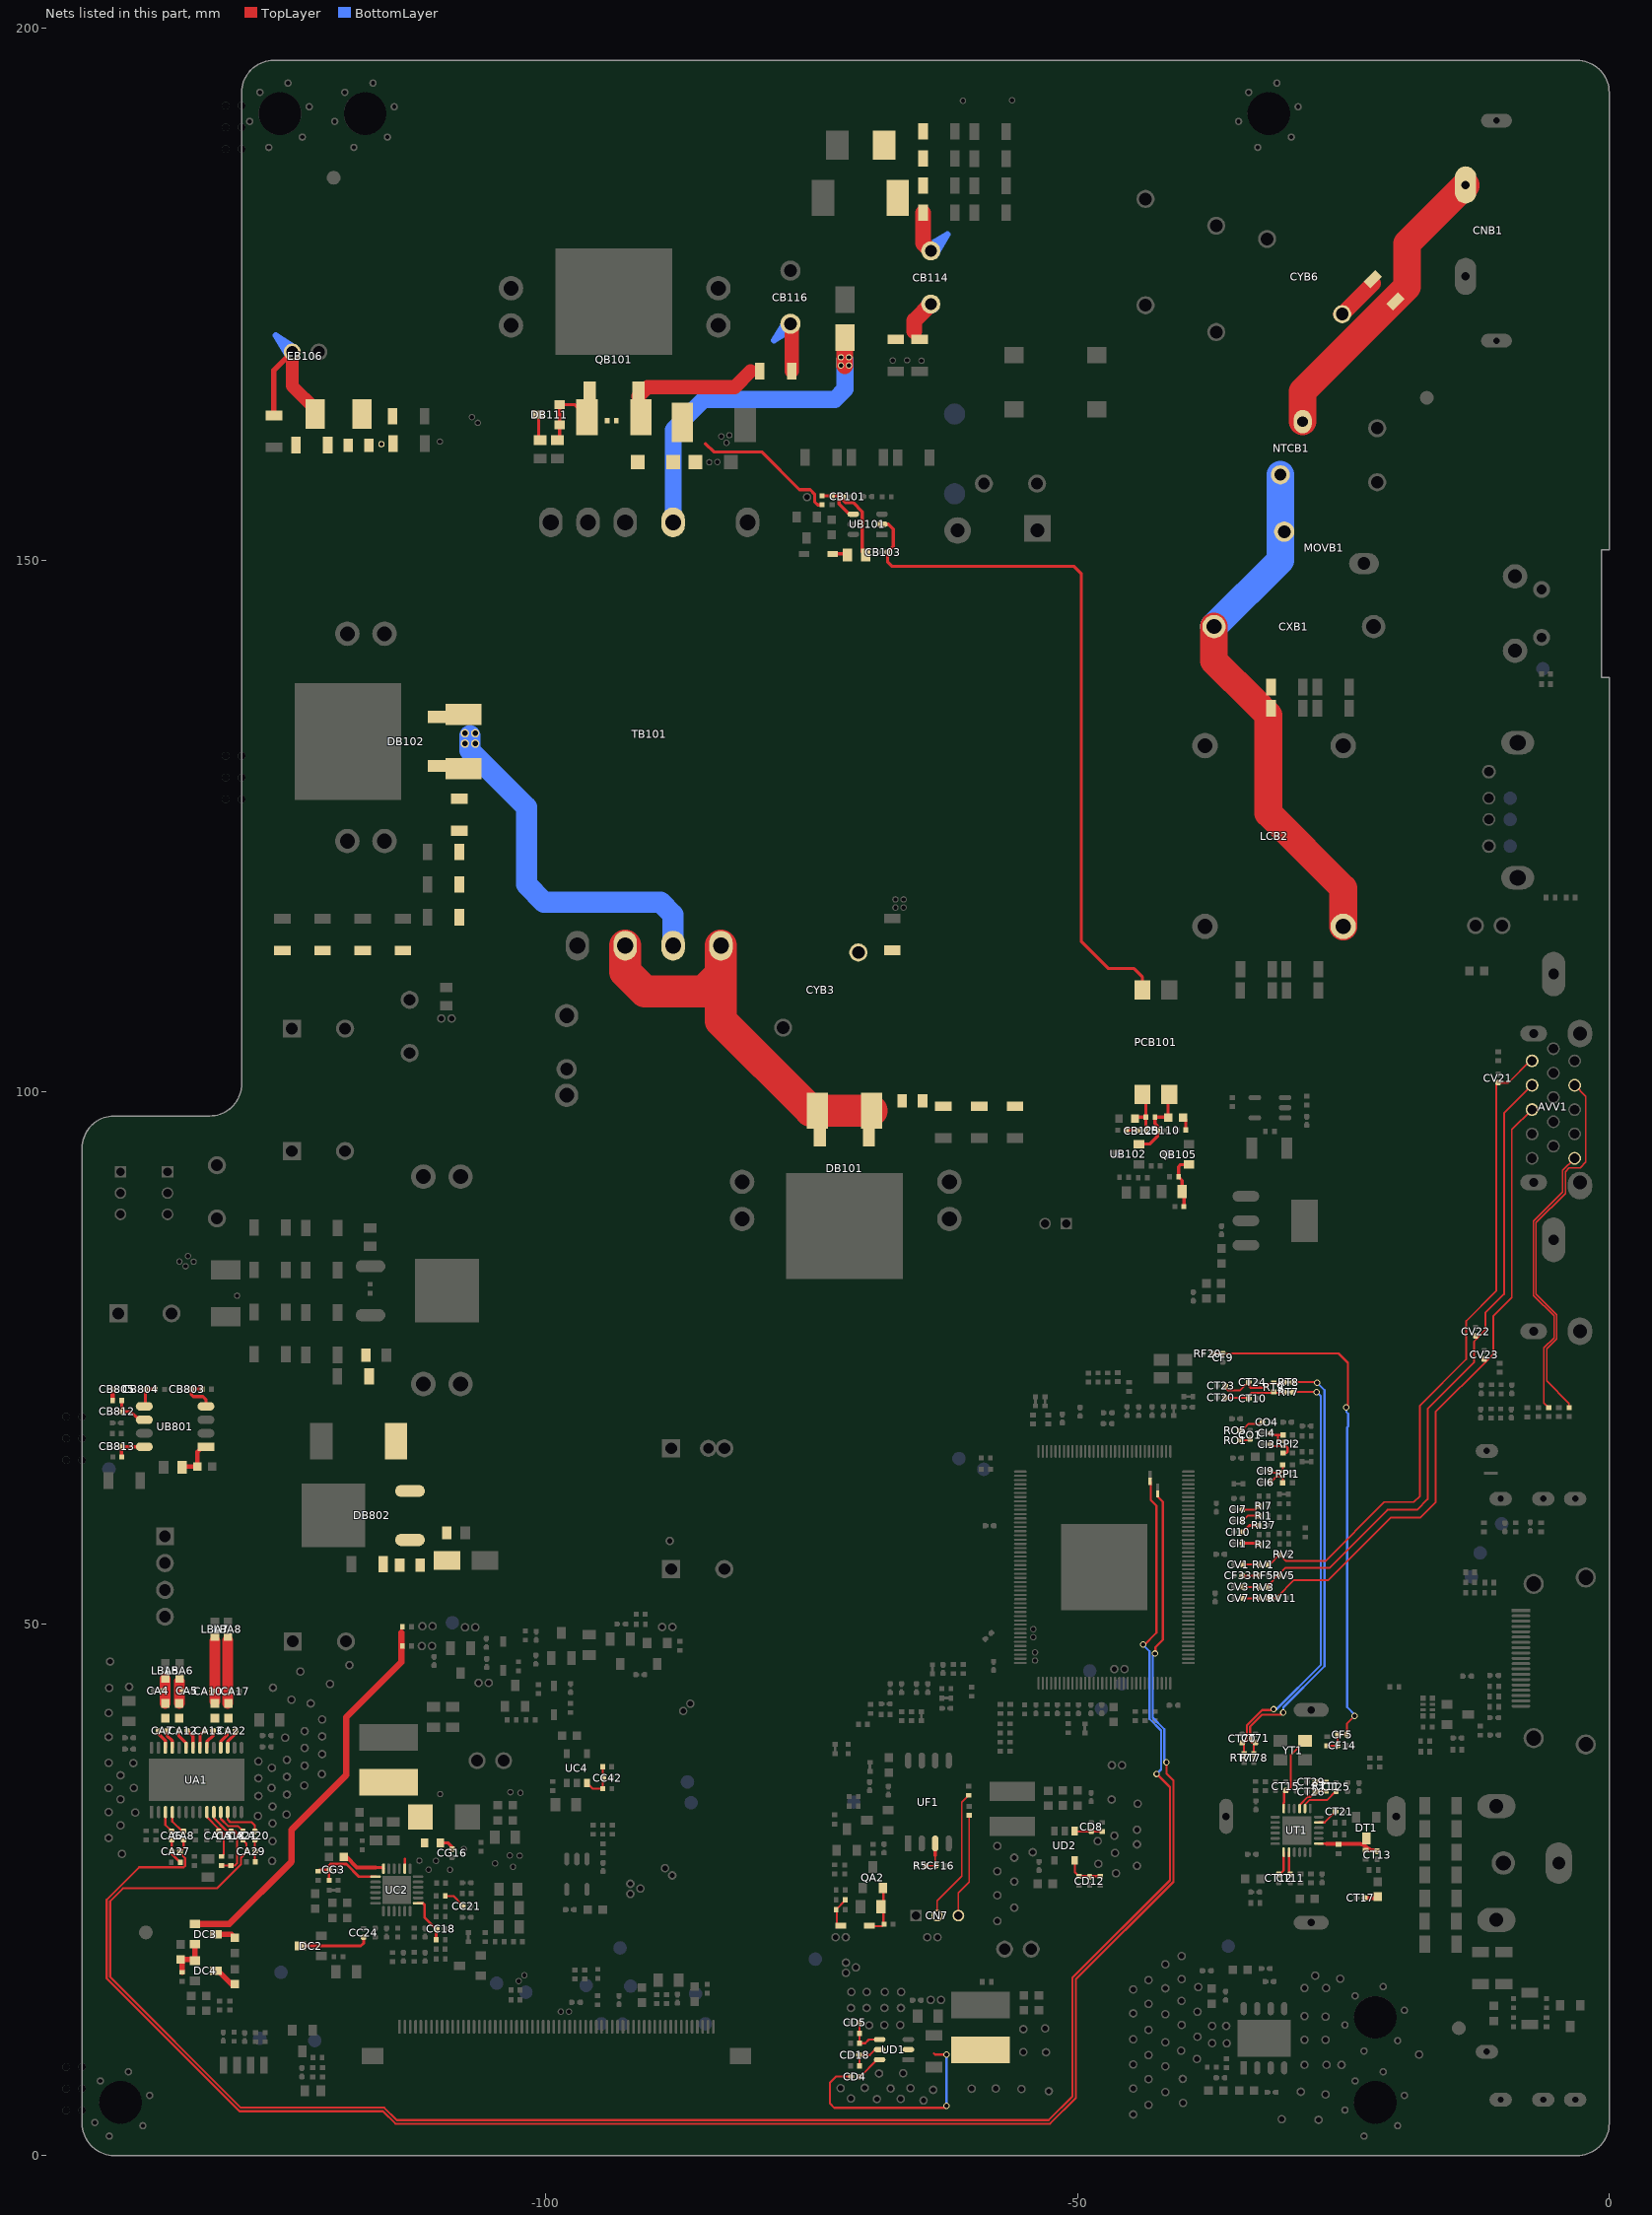
[diagram p0: the nets of this part, all layers, seen from the top]
# Altium PCB MISC86383-9.PcbDoc (part 13 of 18)
Units mm, origin at the board's own origin, x right, y up, seen from the top; angles counter-clockwise.
Board outline 143.6 x 197 mm, 2 copper layers (TopLayer, BottomLayer), stack 1.571 mm thick; 743 components, 401 nets, 2996 pads, 1077 vias.
Unrouted connection lines stored in the file: 4.

## Via types
v1: diameter 0.6, hole 0.4, TopLayer to BottomLayer, tented both sides, 993 vias
v2: diameter 0.6, hole 0.4, TopLayer to BottomLayer, 65 vias
v3: diameter 0.7, hole 0.5, TopLayer to BottomLayer, tented both sides, 15 vias
v4: diameter 0.8, hole 0.5, TopLayer to BottomLayer, tented both sides, 4 vias

## Nets (pads, with @x,y where several pads share a name; then routed paths per layer and width w, separated by ;. In a path a pad name is that pad's centre, name@x,y a point inside that pad or via, vN(x,y) a via of type N, cw(c..) or ccw(c..) an arc to the next point about the centre after c; other vN are vias at no path point) (continued)
N-1: CNB1.2 NTCB1.2@-28.82,163.041 RB160.1 | length 28.7
  TopLayer w2.6: NTCB1.2@-28.82,163.041 -28.82,165.883 -20.237,174.466 -19,175.704 -19,179.8 CNB1.2@-13.572,185.228 ; CNB1.2@-13.572,185.228 CNB1.2@-13.5,185.3 -13.5,185.228 CNB1.2@-13.572,185.228
N-2: CXB1.2 LCB2.1 MOVB1.2@-30.56,152.694 NTCB1.1 RB3.2 RB4.2 | length 50.1
  TopLayer w2.6: CXB1.2@-37.155,143.764 -37.155,140.558 -33.243,136.646 -32.24,135.643 -32.052,135.456 -32.052,126.21 -25.009,119.167 LCB2.1@-25.009,115.579
  BottomLayer w2.6: CXB1.2@-37.155,143.764 -30.92,149.998 -30.92,152.694 NTCB1.1@-30.92,158.041
N-3: CYB6.1 RB160.2 | length 4.2
  TopLayer w1.5: CYB6.1@-25.19,173.147 CYB6.1@-25.103,173.147 RB160.2@-22.219,176.031
NetAVV1_1: AVV1.1 CV21.2@-10.44,100.864 CV21.2@-10.44,101.039 RV1.2 RV2.2 | length 63.4
  TopLayer w0.175: RV1.2@-32.069,55.578 -31.92,55.578 RV2.2@-30.986,56.512 -30.379,55.905 -26.691,55.905 -21.153,61.444 -18.365,61.444 -17.799,62.01 -17.799,70.514 -13.446,74.867 -13.446,78.468 -10.624,81.29 -10.624,100.68 CV21.2@-10.44,100.864 -9.487,100.864 -7.351,103 AVV1.1@-7.351,103.03
  TopLayer w0.18: AVV1.1@-7.351,103.03 AVV1.1@-7.247,103.03
NetAVV1_2: AVV1.2 CV22.2@-12.56,77.22 CV22.2@-12.56,77.045 RV3.2 RV5.2 | length 61.5
  TopLayer w0.175: RV3.2@-32.069,53.444 -32.069,53.628 -31.062,54.635 -30.455,55.242 -26.317,55.242 -20.849,60.71 -18.061,60.71 -17.065,61.706 -17.065,70.21 -12.711,74.563 -12.711,76.531 -12.379,76.864 -11.64,77.603 -11.64,79.235 -9.889,80.986 -9.889,97.998 AVV1.2@-7.247,100.64
NetAVV1_3: AVV1.3 CV23.2@-11.747,74.86 CV23.2@-11.747,75.035 RV9.2 RV11.2 | length 60.6
  TopLayer w0.175: RV9.2@-32.069,52.428 RV11.2@-31.192,52.428 -31.192,52.562 -29.649,54.104 -26.416,54.104 -20.545,59.976 -17.757,59.976 -16.331,61.402 -16.331,69.906 -11.562,74.675 -10.906,75.33 -10.906,78.931 -9.155,80.682 -9.155,96.464 -7.269,98.35 AVV1.3@-7.247,98.35
  TopLayer w0.18: AVV1.3@-7.549,98.45 AVV1.3@-7.247,98.45
NetAVV1_12: AVV1.12 RV23.2 | length 35.4
  TopLayer w0.127: RV23.2@-3.759,70.326 -3.759,70.714 -5.879,72.834 -5.879,75.837 -4.928,76.789 -4.928,79.075 -6.871,81.018 -6.871,87.729 -4.127,90.472 -4.127,92.519 -3.776,92.87 -2.724,92.87 -2.184,93.409 -2.184,99.577 AVV1.12@-3.247,100.64
NetAVV1_15: AVV1.15 RV22.2 | length 26.4
  TopLayer w0.127: RV22.2@-5.69,70.326 -6.133,70.769 -6.133,75.942 -5.182,76.894 -5.182,77.263 ; -5.184,77.263 -5.184,78.971 -7.099,80.887 -7.099,87.86 -4.381,90.577 -4.381,92.636 AVV1.15@-3.247,93.77
NetBB101_2: BB101.2 pad.VIA5@-71.488,168.326 pad.VIA5@-71.488,169.088 pad.VIA5@-72.25,168.326 pad.VIA5@-72.25,169.088 TB101.3 | length 31.9
  TopLayer w1.6: -71.882,168.326 -71.882,169.088 BB101.2@-71.882,170.957
  BottomLayer w1.6: TB101.3@-88.028,153.567 -88.028,162.251 -85.149,165.13 -72.817,165.13 -71.857,166.091 -71.857,168.326 -71.857,168.885
NetBB801_2: BB801.2 BB802.2 CB810.1 DB801.A DB802.1 DB802.3
NetCA4_1: CA4.1 LBA1.2 LBA5.1 | length 2.3
  TopLayer w1.016: LBA1.2@-135.791,42.525 -135.791,43.698 LBA5.1@-135.791,44.821
NetCA5_1: CA5.1 LBA2.2 LBA6.1 | length 2
  TopLayer w1.016: LBA2.2@-134.477,42.525 -134.477,43.673 LBA6.1@-134.477,44.574
NetCA6_1: CA6.1 UA1.3 | length 2
  TopLayer w0.203: UA1.3@-135.77,32.291 -135.77,31.097 CA6.1@-135.182,30.508
NetCA6_2: CA6.2@-135.182,29.658 CA6.2@-135.182,29.833 CA27.1 RA21.2 | length 2.4
  TopLayer w0.203: CA27.1@-135.207,28.598 -135.207,28.374 -134.417,27.584 RA21.2@-134.373,27.584 ; CA27.1@-135.182,28.598 CA6.2@-135.182,29.658
NetCA7_1: CA7.1 UA1.26 | length 1.9
  TopLayer w0.305: CA7.1@-136.47,39.939 -136.47,39.711 -135.77,39.011 UA1.26@-135.77,38.341
NetCA7_2: CA7.2@-135.62,39.939 CA7.2@-135.795,39.939 LBA1.1 UA1.25 | length 1.8
  TopLayer w0.305: CA7.2@-135.62,39.939 -135.62,39.496 -135.12,38.996 UA1.25@-135.12,38.341
NetCA8_1: CA8.1 UA1.4 | length 2.4
  TopLayer w0.203: UA1.4@-135.12,32.291 -135.12,31.417 -134.138,30.435 -134.064,30.361 CA8.1@-134.064,30.333
NetCA8_2: CA8.2@-134.064,29.658 CA8.2@-134.064,29.833 CA27.2@-134.357,28.598 CA27.2@-134.532,28.598 RA2.JP_1K | length 178.7
  TopLayer w0.203: CA8.2@-134.064,29.658 -134.064,28.89 CA27.2@-134.357,28.598 -134.357,28.397 -133.917,27.957 -133.919,27.955 -133.919,27.24 -134.053,27.106 -138.245,27.106 -141.301,24.05 -141.301,16.657 -128.81,4.166 -115.323,4.166 -114.146,2.989 -52.579,2.989 -50.145,5.424 -50.145,16.574 -40.976,25.743 -40.976,35.266 -41.626,35.916 -41.626,36.497 -41.631,36.501 v1(-41.631,36.982) ; v1@-42.743,47.18 v1(-42.728,47.196) -42.666,47.257 -42.666,47.796 -41.966,48.496 -41.966,61.461 -42.456,61.951 RA2.JP_1K@-42.456,62.215
  BottomLayer w0.203: v1(-42.728,47.196) -42.926,46.997 -42.926,41.172 -41.836,40.081 -41.836,37.046 -41.796,37.046 -41.732,36.982 v1(-41.631,36.982)
NetCA10_1: CA10.1 LBA3.2 LBA7.1 | length 5.7
  TopLayer w1.016: LBA3.2@-131.118,42.677 -131.118,43.66 -131.118,48.382
NetCA12_1: CA12.1 UA1.22 | length 1.8
  TopLayer w0.305: CA12.1@-133.69,39.939 -133.17,39.419 UA1.22@-133.17,38.341
NetCA12_2: CA12.2@-134.54,39.939 CA12.2@-134.365,39.939 LBA2.1 UA1.23 | length 1.9
  TopLayer w0.305: CA12.2@-134.54,39.939 -134.54,39.495 -133.82,38.775 UA1.23@-133.82,38.341
NetCA13_1: CA13.1 UA1.21 | length 1.8
  TopLayer w0.305: UA1.21@-132.52,38.341 -132.52,39.52 CA13.1@-132.101,39.939
NetCA13_2: CA13.2@-131.251,39.939 CA13.2@-131.426,39.939 LBA3.1 UA1.20 | length 1.9
  TopLayer w0.305: UA1.20@-131.87,38.341 -131.87,38.925 -131.251,39.543 CA13.2@-131.251,39.939
NetCA15_1: CA15.1 RA11.2 UA1.9 | length 5.1
  TopLayer w0.203: UA1.9@-131.87,32.291 -131.87,31.822 -130.762,30.715 CA15.1@-130.762,30.508 -130.535,30.508 -130.281,30.254 -130.281,28.352 RA11.2@-130.512,28.121
NetCA17_2: CA17.2@-129.63,43.66 CA17.2@-129.455,43.66 LBA4.2 LBA8.1 | length 5.9
  TopLayer w1.016: LBA4.2@-129.899,42.525 -129.899,43.66 LBA8.1@-129.899,48.43
NetCA18_1: CA18.1 RA11.1 RA12.1 UA1.10 | length 7.7
  TopLayer w0.203: UA1.10@-131.22,32.291 -131.22,31.728 -130,30.508 CA18.1@-129.594,30.508 -129.256,30.508 -129.048,30.3 -129.048,27.473 -129.251,27.271 RA12.1@-129.598,27.271 RA11.1@-130.512,27.271
NetCA20_1: CA20.1 UA1.12 | length 4
  TopLayer w0.203: UA1.12@-129.92,32.291 -129.92,31.588 -129.678,31.346 -127.676,31.346 -127.353,31.024 -127.353,30.514 CA20.1@-127.359,30.508
NetCA20_2: CA20.2@-127.359,29.658 CA20.2@-127.359,29.833 CA29.1 RA5.2 | length 2
  TopLayer w0.203: CA20.2@-127.359,29.658 -127.359,28.604 -127.359,27.657 RA5.2@-127.33,27.629
NetCA21_1: CA21.1 UA1.11 | length 3.2
  TopLayer w0.203: UA1.11@-130.57,32.291 -130.57,31.673 -129.859,30.962 -128.93,30.962 CA21.1@-128.476,30.508
NetCA21_2: CA21.2@-128.476,29.658 CA21.2@-128.476,29.833 CA29.2@-127.96,28.604 CA29.2@-128.135,28.604 RA15.JP_1K | length 184.5
  TopLayer w0.178: CA21.2@-128.476,29.658 CA21.2@-128.394,29.658
  TopLayer w0.203: CA21.2@-128.476,29.658 -128.166,29.348 -128.166,28.604 CA29.2@-128.166,28.501 ; CA29.2@-128.135,28.604 -128.135,28.532 CA29.2@-128.166,28.501 ; v1(-43.82,48.065) -43.82,48.003 -43.777,47.96 -43.746,47.991 -42.576,49.161 -42.576,61.093 -43.114,61.631 -43.114,63.33 RA15.JP_1K@-43.18,63.396 ; v1(-42.558,35.877) -41.307,34.626 -41.307,25.879 -50.475,16.711 -50.475,5.56 -52.716,3.319 -114.009,3.319 -115.186,4.496 -128.673,4.496 -140.971,16.794 -140.971,23.913 -139.763,25.121 -130.934,25.121 -128.661,27.393 -128.661,28.006 CA29.2@-128.166,28.501
  BottomLayer w0.203: v1@-43.777,47.96 -43.231,47.414 -43.231,41.046 -42.14,39.955 -42.14,36.295 v1(-42.558,35.877)
NetCA22_1: CA22.1 UA1.17 | length 1.9
  TopLayer w0.305: UA1.17@-129.92,38.341 -129.92,38.932 -129.118,39.733 CA22.1@-129.118,39.939
NetCA22_2: CA22.2@-129.793,39.939 CA22.2@-129.968,39.939 LBA4.1 UA1.18 | length 1.8
  TopLayer w0.305: UA1.18@-130.57,38.341 -130.57,38.917 -129.968,39.518 CA22.2@-129.968,39.939
NetCA36_2: CA36.2 DA1.K QA2.E RA31.2 | length 5
  TopLayer w0.203: DA1.K@-69.584,21.551 -69.567,21.551 -68.387,21.551 RA31.2@-68.242,21.695 ; QA2.E@-68.305,25.157 -68.242,25.095 -68.242,23.398 -68.242,21.754 RA31.2@-68.242,21.695 ; RA31.2@-68.184,21.754 RA31.2@-68.242,21.695
NetCB101_1: CB101.1 RB103.2 RB105.1 RB112.1 UB101.4 | length 11.8
  TopLayer w0.3: RB105.1@-74.016,156.064 -73.076,156.064 RB103.2@-73.01,156.064 ; RB103.2@-73.076,156.076 -73.023,156.076 RB103.2@-73.01,156.064 ; UB101.4@-71.086,154.341 -71.448,154.341 -72.415,155.308 -72.415,155.644 CB101.1@-72.066,155.994 ; RB112.1@-69.911,150.874 RB112.1@-69.911,150.482 -70.233,150.804 -70.233,154.561 -71.095,155.423 -71.844,155.423 -72.066,155.644 CB101.1@-72.066,155.994 ; RB103.2@-73.01,156.064 -72.135,156.064 CB101.1@-72.066,155.994
NetCB103_1: CB103.1 PCB101.4 UB101.2 | length 66.6
  TopLayer w0.3: UB101.2@-68.77,153.391 UB101.2@-68.386,153.391 -67.767,153.391 -67.323,152.946 -67.323,151.315 CB103.1@-67.863,150.774 -67.863,149.863 -67.424,149.424 -50.309,149.424 -49.649,148.764 -49.649,142.411 -49.652,142.408 -49.652,114.17 -47.089,111.608 -44.679,111.608 -43.904,110.833 PCB101.4@-43.904,109.586
NetCB109_1: CB109.1 CB110.1 PCB101.2 RB132.1 UB102.K | length 7.4
  TopLayer w0.3: UB102.K@-44.221,95.11 -43.218,95.11 -42.487,95.841 CB110.1@-42.487,96.393 -42.487,96.818 -42.711,97.042 RB132.1@-42.711,97.638 -41.499,97.638 CB109.1@-41.473,97.612 -41.473,99.677 PCB101.2@-41.364,99.786
NetCB109_2: CB109.2 RB133.2 | length 1.3
  TopLayer w0.3: CB109.2@-40.061,97.612 -39.809,97.36 RB133.2@-39.809,96.444
NetCB113_1: CB113.1 DB104.A pad.VIA5@-115.456,160.922 RB114.1 RB115.1
NetCB113_2: CB113.2 RB116.1
NetCB114_1: CB114.1@-63.792,174.093 RB117.1 RB118.1 | length 3.2
  TopLayer w1.5: -65.341,171.552 -65.341,172.544 CB114.1@-63.792,174.093
NetCB114_2: CB114.2 DB106.K DB107.K RB153.1 RB154.1 RB155.1 RB157.1 | length 3.9
  TopLayer w1.5: RB153.1@-64.517,182.677 -64.517,179.819 CB114.2@-63.792,179.094
NetCB115_1: CB115.1 QB105.B RB182.1 RB183.1 | length 5
  TopLayer w0.3: RB182.1@-39.986,89.23 -39.986,90.457 CB115.1@-40.157,90.627 -40.157,91.686 RB183.1@-40.494,92.024 -40.494,92.983 -40.297,93.18 QB105.B@-39.522,93.18
NetCB116_1: CB116.1 RB119.2 | length 4.5
  TopLayer w1.3: CB116.1@-76.987,172.239 -76.872,172.124 RB119.2@-76.872,167.78
NetCB117_1: CB117.1 DB101.1 DB101.3 TB101.8 TB101.10 | length 37.6
  TopLayer w3: TB101.8@-92.528,113.767 -92.528,111.311 -90.691,109.474 -85.153,109.474 -83.528,111.1 ; TB101.10@-83.528,113.767 -83.528,111.1 ; DB101.1@-69.378,98.248 -69.618,98.248 -74.218,98.248 DB101.3@-74.458,98.248 -75.096,98.248 -83.528,106.68 -83.528,111.1
NetCB117_2: CB117.2 RB128.1 RB129.1 RB165.1
NetCB118_1: CB118.1 DB102.1 DB102.3 pad.VIA5@-106.642,132.766 pad.VIA5@-106.642,133.731 pad.VIA5@-107.607,132.766 pad.VIA5@-107.607,133.731 TB101.9 | length 34.1
  BottomLayer w2: -107.15,133.502 -107.15,132.766 -107.15,132.105 -101.816,126.771 -101.816,119.507 -100.165,117.856 -89.217,117.856 -88.028,116.667 TB101.9@-88.028,113.767
NetCB118_2: CB118.2 RB124.1 RB125.1 RB126.1 RB127.1 RB162.1 RB163.1 RB164.1
NetCB125_1: CB125.1 PCB101.1 RB131.1 RB132.2 | length 4.4
  TopLayer w0.3: RB131.1@-44.589,97.511 -44.462,97.638 RB132.2@-43.561,97.638 ; CB125.1@-43.543,96.368 -43.561,96.386 RB132.2@-43.561,97.638 ; PCB101.1@-43.536,99.67 -43.561,99.644 RB132.2@-43.561,97.638
NetCB125_2: CB125.2@-44.218,96.368 CB125.2@-44.393,96.368 RB158.1 | length 1
  TopLayer w0.3: RB158.1@-45.371,96.418 -44.443,96.418 CB125.2@-44.393,96.368
NetCB801_2: CB801.2 RB816.2 UB801.1 | length 3.8
  TopLayer w0.4: RB816.2@-134.199,64.706 -134.11,64.795 CB801.2@-132.774,64.795 -132.774,66.159 -132.293,66.64 UB801.1@-131.961,66.64
NetCB803_1: CB803.1 RB806.1 UB801.4 | length 3.7
  TopLayer w0.3: RB806.1@-132.308,72.074 CB803.1@-133.312,72.074 -133.312,71.526 -133.147,71.361 -132.232,71.361 -131.961,71.09 UB801.4@-131.961,70.45
NetCB804_1: CB804.1 RB805.1 UB801.5 | length 2.6
  TopLayer w0.3: UB801.5@-137.761,70.45 -137.65,70.562 CB804.1@-137.65,72.06 -136.725,72.06 RB805.1@-136.703,72.038
NetCB805_2: CB805.2@-140.56,72.047 CB805.2@-140.735,72.047 RB804.1 | length 1
  TopLayer w0.4: RB804.1@-140.741,70.98 CB805.2@-140.741,71.996
NetCB809_1: CB809.1 RB810.1
NetCB810_2: CB810.2 RB812.1
NetCB812_2: CB812.2@-139.916,69.952 CB812.2@-140.091,69.952 RB804.2 UB801.6 | length 3.5
  TopLayer w0.3: RB804.2@-139.89,70.98 -139.89,69.977 CB812.2@-139.916,69.952 -139.014,69.952 -138.243,69.18 UB801.6@-137.761,69.18
NetCB813_2: CB813.2@-139.894,66.675 CB813.2@-140.069,66.675 RB813.1 UB801.8 | length 3.1
  TopLayer w0.3: RB813.1@-139.869,65.684 -139.894,65.71 CB813.2@-139.894,66.675 -139.859,66.64 UB801.8@-137.761,66.64
NetCC11_1: CC11.1 UC2.24 | length 4.2
  TopLayer w0.254: -115.989,27.089 -115.38,27.089 UC2.24@-115.264,26.973
  TopLayer w0.381: CC11.1@-118.991,28.092 -118.758,28.092 -117.754,27.089 -115.989,27.089
NetCC18_2: CC18.2@-110.134,21.302 CC18.2@-110.309,21.302 RC14.1 UC2.13 | length 4.5
  TopLayer w0.254: UC2.13@-112.014,23.723 -111.543,23.723 -111.403,23.584 -111.403,22.397 CC18.2@-110.309,21.302 -110.309,20.308 RC14.1@-110.305,20.304 ; RC14.1@-110.318,20.253 -110.309,20.262 RC14.1@-110.309,20.302
NetCC21_1: CC21.1 RC13.2 | length 2.1
  TopLayer w0.203: RC13.2@-109.459,24.401 -108.691,24.401 -107.868,23.579 CC21.1@-107.868,23.463 CC21.1@-107.931,23.401
NetCC24_2: CC24.2@-117.129,20.512 CC24.2@-117.129,20.687 DC2.2 | length 6.6
  TopLayer w0.254: DC2.2@-123.083,19.704 -117.392,19.704 -117.129,19.967 CC24.2@-117.129,20.512
NetCC27_1: CC27.1 DC3.2 | length 1.9
  TopLayer w0.508: DC3.2@-131.011,20.816 -129.583,20.816 CC27.1@-129.235,20.468
NetCC31_1: CC31.1 DC4.2 | length 2.3
  TopLayer w0.508: DC4.2@-131.023,17.368 -130.817,17.368 -129.558,16.108 CC31.1@-129.269,16.108
NetCC42_1: CC42.1 RC31.2 RC35.1 UC4.3 | length 3.8
  TopLayer w0.203: UC4.3@-96.129,35.036 -95.586,34.493 RC35.1@-94.633,34.493 CC42.1@-94.633,35.496 ; RC31.2@-94.646,36.551 -94.633,36.538 CC42.1@-94.633,35.496
NetCD4_1: CD4.1 LD1.1 UD1.2 | length 21.6
  TopLayer w0.203: CD4.1@-71.342,7.417 -72.72,7.417 -73.279,6.858 -73.279,4.894 -72.873,4.488 -62.407,4.488 -62.315,4.58 v1(-62.315,4.661) ; -63.51,9.613 -63.396,9.499 v1(-62.308,9.499) v1@-62.159,9.499
  BottomLayer w0.203: v1(-62.315,4.661) -62.315,9.492 v1(-62.308,9.499)
NetCD4_2: CD4.2@-70.492,7.417 CD4.2@-70.667,7.417 UD1.6 | length 2.5
  TopLayer w0.203: CD4.2@-70.492,7.417 -70.434,7.417 -68.844,9.007 UD1.6@-68.609,9.007
NetCD5_1: CD5.1 RD3.1 RD5.2 UD1.4 | length 4
  TopLayer w0.203: CD5.1@-70.494,12.49 RD3.1@-70.493,11.474 RD5.2@-70.493,10.56 -69.958,10.56 -69.611,10.907 UD1.4@-68.609,10.907
NetCD8_2: CD8.2@-48.701,30.464 CD8.2@-48.701,30.639 RD7.1 UD2.1 | length 2.6
  TopLayer w0.203: UD2.1@-50.249,30.507 -50.214,30.472 -48.701,30.472 RD7.1@-47.689,30.472
NetCD12_1: CD12.1 RD8.1 RD9.2 UD2.5 | length 3.7
  TopLayer w0.203: UD2.5@-50.249,27.757 -50.249,26.643 RD8.1@-49.873,26.267 ; RD8.1@-49.851,26.245 RD8.1@-49.873,26.267 ; RD9.2@-47.84,26.245 -47.853,26.257 -47.862,26.267 -47.865,26.267 -48.854,26.267 -49.851,26.267 RD8.1@-49.873,26.267
NetCD18_2: CD18.2@-70.67,9.451 CD18.2@-70.495,9.451 RD1.2 UD1.5 | length 3.1
  TopLayer w0.203: RD1.2@-70.495,8.435 CD18.2@-70.495,9.451 -69.543,9.451 -69.037,9.957 UD1.5@-68.609,9.957
NetCF5_1: CF5.1 CF9.2@-36.332,75.261 CF9.2@-36.332,75.436 RF20.2 | length 48.9
  TopLayer w0.203: RF20.2@-37.33,75.417 -36.332,75.417 -25.455,75.417 -24.569,74.531 -24.569,70.337 v1(-24.722,70.337) ; CF5.1@-24.671,39.563 -24.671,40.595 v1(-23.929,41.337)
  BottomLayer w0.203: v1(-24.722,70.337) -24.722,69.917 -24.544,69.74 -24.544,68.559 -24.642,68.462 -24.642,67.834 -24.642,42.634 ; -24.642,42.598 -24.642,42.168 -23.929,41.455 v1(-23.929,41.337)
NetCF5_2: CF5.2 CF5.3 CF14.2@-25.36,38.547 CF14.2@-25.535,38.547 LF1.1 | length 2
  TopLayer w0.203: LF1.1@-26.52,38.541 -25.541,38.541 CF14.2@-25.535,38.547 CF5.2@-25.535,39.563
NetCF16_1: CF16.1 R5.1 UF1.3 | length 3.1
  TopLayer w0.127: R5.1@-64.287,27.254 CF16.1@-63.308,27.254 -63.376,27.322 -63.376,28.219
  TopLayer w0.305: -63.376,28.219 UF1.3@-63.376,29.342
NetCF33_2: CF33.2@-34.466,54.523 CF33.2@-34.641,54.523 RF5.1 | length 1.6
  TopLayer w0.175: CF33.2@-34.466,54.523 -33.11,54.523 -32.995,54.638 RF5.1@-32.919,54.714
NetCG3_1: CG3.1 RG15.1 RG16.2 UC2.1 | length 7.4
  TopLayer w0.254: RG15.1@-121.405,26.732 -121.259,26.878 CG3.1@-120.382,26.878 ; RG16.2@-120.378,25.875 -120.378,26.874 CG3.1@-120.382,26.878 ; UC2.1@-116.014,26.223 -117.587,26.223 -118.758,27.394 -120.244,27.394 -120.382,27.255 CG3.1@-120.382,26.878
NetCG16_2: CG16.2@-108.814,28.86 CG16.2@-108.814,28.685 RG82.1 | length 1.3
  TopLayer w0.305: RG82.1@-109.899,29.4 -109.22,29.4 -108.814,28.994 CG16.2@-108.814,28.899
NetCG28_1: CG28.1 DC3.3 DC4.1 RC23.1 | length 4.2
  TopLayer w0.508: RC23.1@-134.212,17.228 -134.212,18.291 CG28.1@-134.353,18.433 -133.117,18.433 DC4.1@-133.005,18.321 -132.993,18.333 DC3.3@-132.993,19.863
NetCI1_2: CI1.2@-34.457,57.571 CI1.2@-34.632,57.571 RI2.2 | length 1.6
  TopLayer w0.254: CI1.2@-34.457,57.571 -32.996,57.571 RI2.2@-32.907,57.483
NetCI3_2: CI3.2@-31.778,66.874 CI3.2@-31.953,66.874 RPI2.5 RPI2.7 | length 2.5
  TopLayer w0.203: CI3.2@-31.778,66.874 -31.613,66.709 -30.724,66.709 RPI2.5@-30.671,66.656 -30.663,66.665 -30.336,66.665 -30.25,66.579 -30.25,66.153 -30.347,66.056 RPI2.7@-30.671,66.056
NetCI4_2: CI4.2@-31.778,67.935 CI4.2@-31.953,67.935 RPI2.1 RPI2.3 | length 2.3
  TopLayer w0.203: CI4.2@-31.953,67.783 -31.942,67.772 -31.926,67.756 -31.778,67.756 -31.174,67.756 ; RPI2.3@-30.671,67.156 -31.005,67.156 -31.136,67.287 -31.136,67.718 -31.174,67.756 ; RPI2.1@-30.671,67.756 -31.174,67.756
NetCI6_2: CI6.2@-31.842,63.29 CI6.2@-32.017,63.29 RPI1.5 RPI1.7 | length 2
  TopLayer w0.203: CI6.2@-31.842,63.29 -31.283,63.849 RPI1.5@-30.697,63.849 RPI1.7@-30.697,63.249 RPI1.7@-30.738,63.29
NetCI7_2: CI7.2@-34.457,60.734 CI7.2@-34.632,60.734 RI7.1 | length 1.7
  TopLayer w0.178: CI7.2@-34.457,60.734 -33.25,60.734 RI7.1@-32.907,61.077
NetCI8_2: CI8.2@-34.457,59.705 CI8.2@-34.632,59.705 RI1.2 | length 1.7
  TopLayer w0.18: CI8.2@-34.457,59.705 -34,60.162 RI1.2@-32.907,60.162
NetCI9_2: CI9.2@-31.842,64.357 CI9.2@-32.017,64.357 RPI1.1 RPI1.3 | length 1.8
  TopLayer w0.178: CI9.2@-31.842,64.205 -31.832,64.215 -30.831,64.215 RPI1.3@-30.697,64.349 RPI1.1@-30.697,64.949
NetCI10_2: CI10.2@-34.457,58.638 CI10.2@-34.632,58.638 RI37.1 | length 1.8
  TopLayer w0.254: CI10.2@-34.457,58.638 -33.848,59.248 RI37.1@-32.907,59.248
NetCN7_2: CN7.2 RV21.1 | length 12.5
  TopLayer w0.127: CN7.2@-63.195,22.555 -63.195,23.95 -60.861,26.284 -60.861,33.227 RV21.1@-60.223,33.865
NetCN7_3: CN7.3 RV20.1 | length 9.8
  TopLayer w0.127: CN7.3@-61.195,22.555 -61.195,24.708 -60.198,25.705 RV20.1@-60.198,31.985
NetCO1_2: CO1.2@-33.752,67.344 CO1.2@-33.752,67.519 RO1.2 | length 0.9
  TopLayer w0.178: RO1.2@-34.749,67.262 -33.936,67.262 CO1.2@-33.853,67.344
NetCO4_2: CO4.2@-32.458,68.951 CO4.2@-32.633,68.951 RO5.2 | length 2.4
  TopLayer w0.178: RO5.2@-34.749,68.189 -34.513,68.189 -33.906,68.796 -32.788,68.796 CO4.2@-32.633,68.951
NetCT10_1: CT10.1 CT20.1 RT7.2 RT7.3 RT9.1 | length 5.7
  TopLayer w0.203: CT20.1@-36.062,71.26 -34.074,71.26 -33.621,71.713 RT7.2@-30.668,71.713
  TopLayer w0.305: RT7.2@-30.668,71.713 RT7.2@-30.588,71.794
NetCT11_2: CT11.2@-29.987,26.313 CT11.2@-29.987,26.488 UT1.20 | length 2.1
  TopLayer w0.203: UT1.20@-30.11,28.52 -30.11,26.61 CT11.2@-29.987,26.488
NetCT12_1: CT12.1 UT1.19 | length 2.2
  TopLayer w0.203: CT12.1@-30.915,26.487 -30.61,26.793 UT1.19@-30.61,28.52
NetCT13_2: CT13.2@-21.831,28.49 CT13.2@-21.831,28.665 DT1.2 LT3.2 LT6.1 UT1.1 | length 5.7
  TopLayer w0.229: UT1.1@-27.31,29.32 -26.561,29.32
  TopLayer w0.368: -26.561,29.32 -25.435,29.32 -23.587,29.32 cw(c-23.587,28.301) -22.867,29.022 ccw(c-22.005,29.884) -22.005,28.665 CT13.2@-21.831,28.665
NetCT15_2: CT15.2@-30.414,34.46 CT15.2@-30.414,34.285 UT1.12 YT1.3 | length 7.1
  TopLayer w0.203: UT1.12@-30.61,32.62 -30.61,33.16 -30.57,33.2 CT15.2@-30.57,34.129 ; CT15.2@-30.414,34.285 -30.23,34.285 -29.935,34.581 -29.935,37.675 YT1.3@-28.608,39.002
NetCT17_1: CT17.1 LT9.2 | length 1.2
  TopLayer w0.368: CT17.1@-22.949,24.216 -21.867,24.216 LT9.2@-21.75,24.333
NetCT21_1: CT21.1 UT1.5 | length 2
  TopLayer w0.203: UT1.5@-27.31,31.32 -26.769,31.32 -25.842,32.247 -25.797,32.247 CT21.1@-25.728,32.247
NetCT23_1: CT23.1 CT24.2@-33.771,72.721 CT24.2@-33.946,72.721 RT8.2 RT8.3 RT9.2 | length 6.5
  TopLayer w0.203: CT23.1@-36.062,72.168 -35.828,71.933 -34.734,71.933 CT24.2@-33.946,72.721 -33.846,72.62 -33.846,72.321 -33.716,72.191 -32.33,72.191 -31.947,72.574 -30.734,72.574 RT8.2@-30.588,72.721
NetCT25_1: CT25.1 UT1.8 | length 3.8
  TopLayer w0.191: UT1.8@-28.61,32.62 -28.61,33.006 -28.202,33.413 -26.537,33.413 CT25.1@-25.728,34.223
NetCT26_2: CT26.2@-27.601,34.203 CT26.2@-27.776,34.203 RT11.2 UT1.9 | length 3.3
  TopLayer w0.191: UT1.9@-29.11,32.62 -29.11,32.955 -28.334,33.73 -28.073,33.73 -27.689,34.115 CT26.2@-27.601,34.203 -27.53,34.273 RT11.2@-26.642,34.273
NetCT29_2: CT29.2@-27.601,35.13 CT29.2@-27.776,35.13 RT11.1 | length 1
  TopLayer w0.191: CT29.2@-27.601,35.13 -26.649,35.13 RT11.1@-26.642,35.123
NetCT70_1: CT70.1 RT7.1 RT77.2 RT77.3 | length 40.4
  TopLayer w0.203: RT77.2@-34.337,37.809 -34.337,38.597 CT70.1@-34.52,38.779 -34.324,38.779 -34.067,39.036 -34.067,40.46 -32.64,41.887 -31.561,41.887 v1(-31.561,41.963) ; RT7.1@-29.738,71.794 -27.516,71.794 v1(-27.51,71.787)
  BottomLayer w0.203: v1(-31.561,41.963) -31.285,41.963 -27.106,46.142 -27.106,71.384 v1(-27.51,71.787)
NetCT71_2: CT71.2@-33.266,38.804 CT71.2@-33.266,38.979 RT8.1 RT78.2 RT78.3 | length 41.5
  TopLayer w0.203: RT78.2@-33.419,37.809 -33.419,38.652 CT71.2@-33.266,38.804 -33.567,38.804 -33.762,38.999 -33.762,40.334 -32.639,41.457 v1@-30.848,41.457 ; RT8.1@-29.738,72.721 -27.531,72.721 v1(-27.47,72.66)
  BottomLayer w0.203: v1(-30.647,41.658) -30.647,42.134 -26.776,46.005 -26.776,71.966 v1(-27.47,72.66)
NetCV1_2: CV1.2@-34.458,55.547 CV1.2@-34.633,55.547 RV1.1 | length 1.6
  TopLayer w0.175: CV1.2@-34.458,55.547 -34.427,55.578 RV1.1@-32.919,55.578
NetCV3_2: CV3.2@-34.458,53.464 CV3.2@-34.633,53.464 RV3.1 | length 1.5
  TopLayer w0.178: CV3.2@-34.458,53.464 -32.939,53.464 RV3.1@-32.919,53.444
NetCV7_2: CV7.2@-34.62,52.397 CV7.2@-34.445,52.397 RV9.1 | length 1.5
  TopLayer w0.175: CV7.2@-34.445,52.397 -32.95,52.397 RV9.1@-32.919,52.428
NetCYB3_1: CYB3.1 RB130.2
NetDA1_A: DA1.A RA16.2 RA18.2 | length 3
  TopLayer w0.203: DA1.A@-72.636,21.449 -72.636,21.615 -72.636,23.056 RA18.2@-72.705,23.125 -71.855,23.975 RA16.2@-71.855,24.04
NetDB104_K: DB104.K EB106.1 RB110.2 RB116.2 | length 13.4
  TopLayer w0.5: RB110.2@-125.565,163.616 -125.565,167.861 EB106.1@-123.843,169.583
  TopLayer w1.2: EB106.1@-123.843,169.583 -123.843,166.388 -121.694,164.239 DB104.K@-121.694,163.767
NetDB109_A: DB109.A QB101.3 RB105.2 RB109.1 RB119.1 RB148.2 | length 26.4
  TopLayer w0.3: RB148.2@-87.151,161.865 RB148.2@-87.151,162.979 ; -84.976,160.96 -84.213,160.197 -79.702,160.197 -76.15,156.646 -75.134,156.646 -74.723,156.234 -74.723,155.508 -74.429,155.213 RB105.2@-74.016,155.213
  TopLayer w1.3: QB101.3@-91.288,165.411 -91.287,165.412 -90.418,166.281 -82.22,166.281 -80.721,167.78
NetDB109_K: DB109.K DB110.A
NetDB111_1: DB111.1 DB111.3 QB101.1 RB106.2 RB109.2 | length 6.7
  TopLayer w0.3: RB106.2@-98.92,161.305 -98.692,161.534 DB111.1@-98.692,162.738 DB111.3@-98.692,164.643 ; DB111.3@-98.869,164.643 DB111.3@-98.692,164.643 ; QB101.1@-96.128,163.461 -97.31,164.643 DB111.3@-98.692,164.643
NetDB111_2: DB111.2 RB107.2 | length 2.5
  TopLayer w0.3: DB111.2@-100.674,163.69 -100.674,161.42 RB107.2@-100.546,161.292
NetDB112_K: DB112.K RB112.2 | length 1.4
  TopLayer w0.3: DB112.K@-73.021,150.609 -71.77,150.609 RB112.2@-71.643,150.482
NetDC1_A: DC1.A LC1.2 RG82.2 UC2.20 | length 0.9
  TopLayer w0.254: UC2.20@-113.264,26.973 -113.264,27.882
NetDC3_1: DC3.1 RC19.1 RC20.2 | length 37.3
  TopLayer w0.61: DC3.1@-132.993,21.768 -129.774,21.768 -123.901,27.642 -123.901,30.639 -118.783,35.756 -118.783,41.186 -113.589,46.38 -113.589,47.904 -113.589,49.174